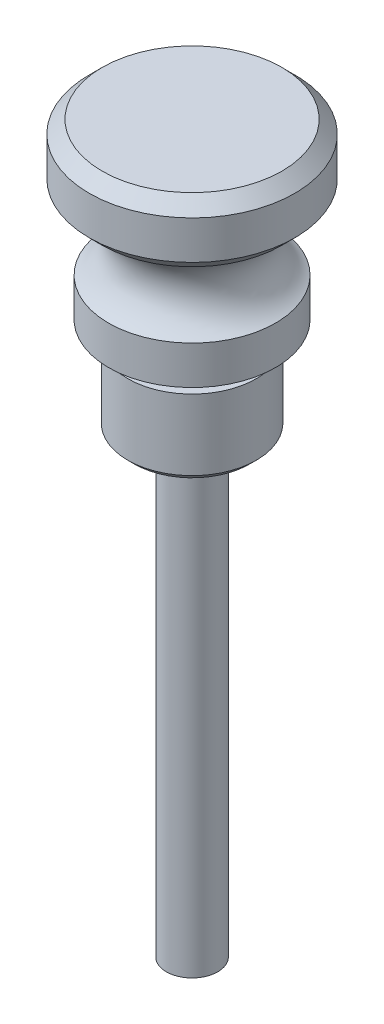
from build123d import *

# Parameters (mm, degrees)
SCALE_1_SCALE = 1.875


with BuildPart() as part:
    # Sketch1 → Revolve1 (revolve)
    with BuildSketch(Plane.XY, mode=Mode.PRIVATE) as revolve1_sk:
        with BuildLine():
            Line((4, -40), (4, -111))
            Line((4, -111), (2, -112))
            Line((2, -112), (0, -112))
            Line((0, -112), (0, 2))
            Line((0, 2), (14, 2))
            Line((14, 2), (16, 0))
            Line((16, 0), (16, -6))
            Line((16, -6), (14, -8))
            ThreePointArc((14, -8), (9.860217357, -13.169110669), (13, -19))
            Line((13, -19), (13, -25))
            Line((13, -25), (6.5, -25))
            Line((6.5, -25), (6.5, -28))
            Line((6.5, -28), (10, -28))
            Line((10, -28), (10, -39))
            Line((10, -39), (9, -40))
            Line((9, -40), (4, -40))
        make_face()
    revolve(revolve1_sk.sketch.rotate(Axis((0, 2, 0), (0, -1, 0)), 90), axis=Axis((0, 2, 0), (0, -1, 0)))


with BuildPart() as part_1:
    # Scale 1: scaled about (0, -24.610702711, 0)
    add(part.part.scale(SCALE_1_SCALE).moved(Location((0, 21.534364872, 0))))


solid = part_1.part
